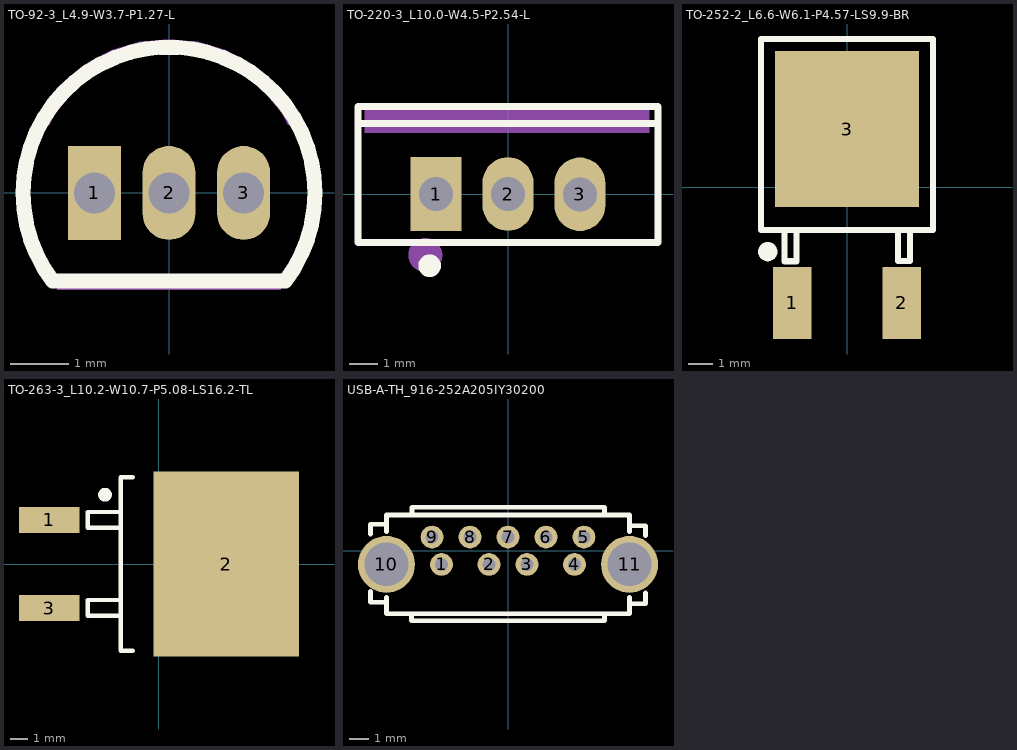
[diagram p0: the footprints below, top view; thin cyan lines are the x and y axes]
# Altium footprint library MISC84402-2.PcbLib: 69 footprints (part 5 of 5)
Each footprint in its own frame and in the unit in brackets; x right, y up, seen from the top. Pads: shape width x height; smd on the part's side, far side on the other; paste and mask are expansions set on the pad; w line width, h text height; cw(c..) or ccw(c..) is an arc to the next point about the centre after c.

## TO-92-3_L4.9-W3.7-P1.27-L [mm]
pads (3):
  rect 0.9x1.6 hole 0.7: 1(-1.27,0)
  oval 0.9x1.6 hole 0.7: 2(0,0) 3(1.27,0)
Top Overlay:
  lines w0.254: -1.981,-1.501 cw(c0,-0.003) 1.981,-1.501 ; -1.98,-1.5 1.98,-1.5
Mechanical 15:
  region: -1.905,-1.397 1.905,-1.397 1.905,-1.651 -1.905,-1.651
  region: -2.29,1.16 -2.036,1.16 -1.926,1.367 -1.638,1.717 -1.288,2.004 -0.888,2.218 -0.455,2.349 -0.004,2.394 0.447,2.349 0.88,2.218 1.28,2.004 1.63,1.717 1.918,1.367 2.028,1.16 2.282,1.16 2.16,1.417 2.127,1.481 1.808,1.869 1.42,2.188 0.977,2.424 0.496,2.57 -0.004,2.619 -0.504,2.57 -0.985,2.424 -1.428,2.188 -1.816,1.869 -2.135,1.481 -2.168,1.417 -2.163,1.414

## TO-220-3_L10.0-W4.5-P2.54-L [mm]
pads (3):
  rect 1.8x2.6 hole 1.2: 1(-2.54,0.005)
  oval 1.8x2.6 hole 1.2: 2(0,0.005) 3(2.54,-0.005)
Top Overlay:
  lines w0.254: -5.3,2.495 5.3,2.495 ; -5.301,-1.704 5.301,-1.704 5.301,3.094 -5.301,3.094 -5.301,3.089 -5.301,-1.704
  lines w0.4: -2.77,-2.33 ccw(c-2.769,-2.53) -2.768,-2.33
Mechanical 15:
  circle w0.6: c-2.921,-2.154 r0.3
  region: -5.06,3.01 -5.06,2.17 4.99,2.17 4.99,3.01

## TO-252-2_L6.6-W6.1-P4.57-LS9.9-BR [mm]
pads (3):
  rect 1.6x3 smd: 1(-2.285,-4.806) 2(2.285,-4.8)
  rect 6x6.5 smd: 3(0,2.428)
Top Overlay:
  lines w0.254: -2.6,-1.771 -2.6,-3.071 -2.1,-3.071 -2.1,-1.771 ; 2.122,-1.767 2.122,-3.067 2.623,-3.067 2.623,-1.767 ; -3.573,-1.771 3.573,-1.771 3.573,6.179 -3.573,6.179 -3.573,-1.771
  lines w0.4: -3.099,-2.674 cw(c-3.299,-2.672) -3.099,-2.671
Mechanical 15:
  circle w0.4: c-2.337,-4.44 r0.2

## TO-263-3_L10.2-W10.7-P5.08-LS16.2-TL [mm]
pads (3):
  rect 3.504x1.5 smd: 1(-6.326,2.54) 3(-6.326,-2.54)
  rect 8.38x10.7 smd: 2(3.888,0)
Top Overlay:
  lines w0.254: -2.213,-2.98 -4.113,-2.98 -4.113,-2.08 -2.213,-2.08 ; -2.213,2.1 -4.113,2.1 -4.113,3 -2.213,3 ; -1.513,-5 -2.213,-5 -2.213,5 -1.513,5
  lines w0.4: -3.115,3.8 cw(c-3.114,4) -3.113,3.8

## USB-A-TH_916-252A205IY30200 [mm]
pads (11):
  round 1.2 hole 0.7: 1(-3.5,-0.72) 2(-1,-0.72) 3(1,-0.72) 4(3.5,-0.72) 5(4,0.72) 6(2,0.72) 7(0,0.72) 8(-2,0.72) 9(-4,0.72)
  round 3 hole 2.3: 10(-6.4,-0.72) 11(6.4,-0.72)
Top Overlay:
  lines w0.254: -7.239,-2.149 -7.239,-2.709 -6.4,-2.709 ; -7.239,0.879 -7.239,1.397 -6.4,1.397 ; -6.4,-2.451 -6.4,-3.32 6.4,-3.32 6.4,-2.451 ; -6.4,1.011 -6.4,1.88 6.4,1.88 6.4,1.011 ; -5.08,-3.32 -5.08,-3.683 5.08,-3.683 5.08,-3.32 ; -5.055,1.88 -5.055,2.286 5.08,2.286 5.08,1.88 ; 6.4,-2.794 7.239,-2.794 7.239,-2.234 ; 6.4,1.312 7.239,1.312 7.239,0.794